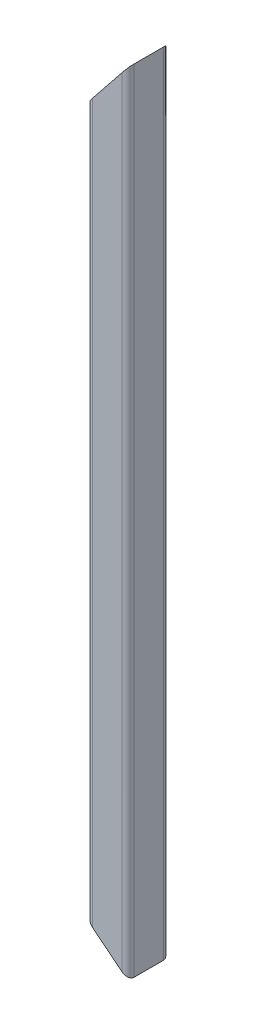
from build123d import *

# Parameters (mm, degrees)
FEATURE_19_WELDMEMBERFEAT_4_MORE_IN_5_DEPTH = 1340
CUT_EXTRUDE1_DEPTH                          = 1343.283502096
CUT_EXTRUDE1_DEPTH_BACK                     = 1343.283502096


with BuildPart() as part:
    # Sketch1 → feature 19 (WeldMemberFeat) (+4 more in 5 files) Cold-formed Hollow Structural Square Steel(gb t6728-2002) 70×70×5(1) (new body)
    with BuildSketch(Plane(origin=(0, 0, 0), x_dir=(-1, 0, 0), z_dir=(0, 1, 0))):
        with BuildLine():
            Line((-25, -35), (25, -35))
            ThreePointArc((25, -35), (32.071067812, -32.071067812), (35, -25))
            Line((35, -25), (35, 25))
            ThreePointArc((35, 25), (32.071067812, 32.071067812), (25, 35))
            Line((25, 35), (-25, 35))
            ThreePointArc((-25, 35), (-32.071067812, 32.071067812), (-35, 25))
            Line((-35, 25), (-35, -25))
            ThreePointArc((-35, -25), (-32.071067812, -32.071067812), (-25, -35))
        make_face()
        with BuildLine():
            Line((-25, -30), (25, -30))
            ThreePointArc((25, -30), (28.535533906, -28.535533906), (30, -25))
            Line((30, -25), (30, 25))
            ThreePointArc((30, 25), (28.535533906, 28.535533906), (25, 30))
            Line((25, 30), (-25, 30))
            ThreePointArc((-25, 30), (-28.535533906, 28.535533906), (-30, 25))
            Line((-30, 25), (-30, -25))
            ThreePointArc((-30, -25), (-28.535533906, -28.535533906), (-25, -30))
        make_face(mode=Mode.SUBTRACT)
    extrude(amount=FEATURE_19_WELDMEMBERFEAT_4_MORE_IN_5_DEPTH)

    # 0:feat:20/0 feature 20/0 (ProfileFeature) (+11 more in 7 files) Sketch2 → Cut-Extrude1 (cut, two sides: drawn at the far end of the back side and taken through both)
    with BuildSketch(Plane.XY.offset(35).offset(-CUT_EXTRUDE1_DEPTH_BACK)):
        Polygon((35, 1340), (-35, 1252.5), (-35, 1340), align=None)
        Polygon((-35, 56), (35, 0), (-35, 0), align=None)
    extrude(amount=CUT_EXTRUDE1_DEPTH + CUT_EXTRUDE1_DEPTH_BACK, mode=Mode.SUBTRACT)


solid = part.part
